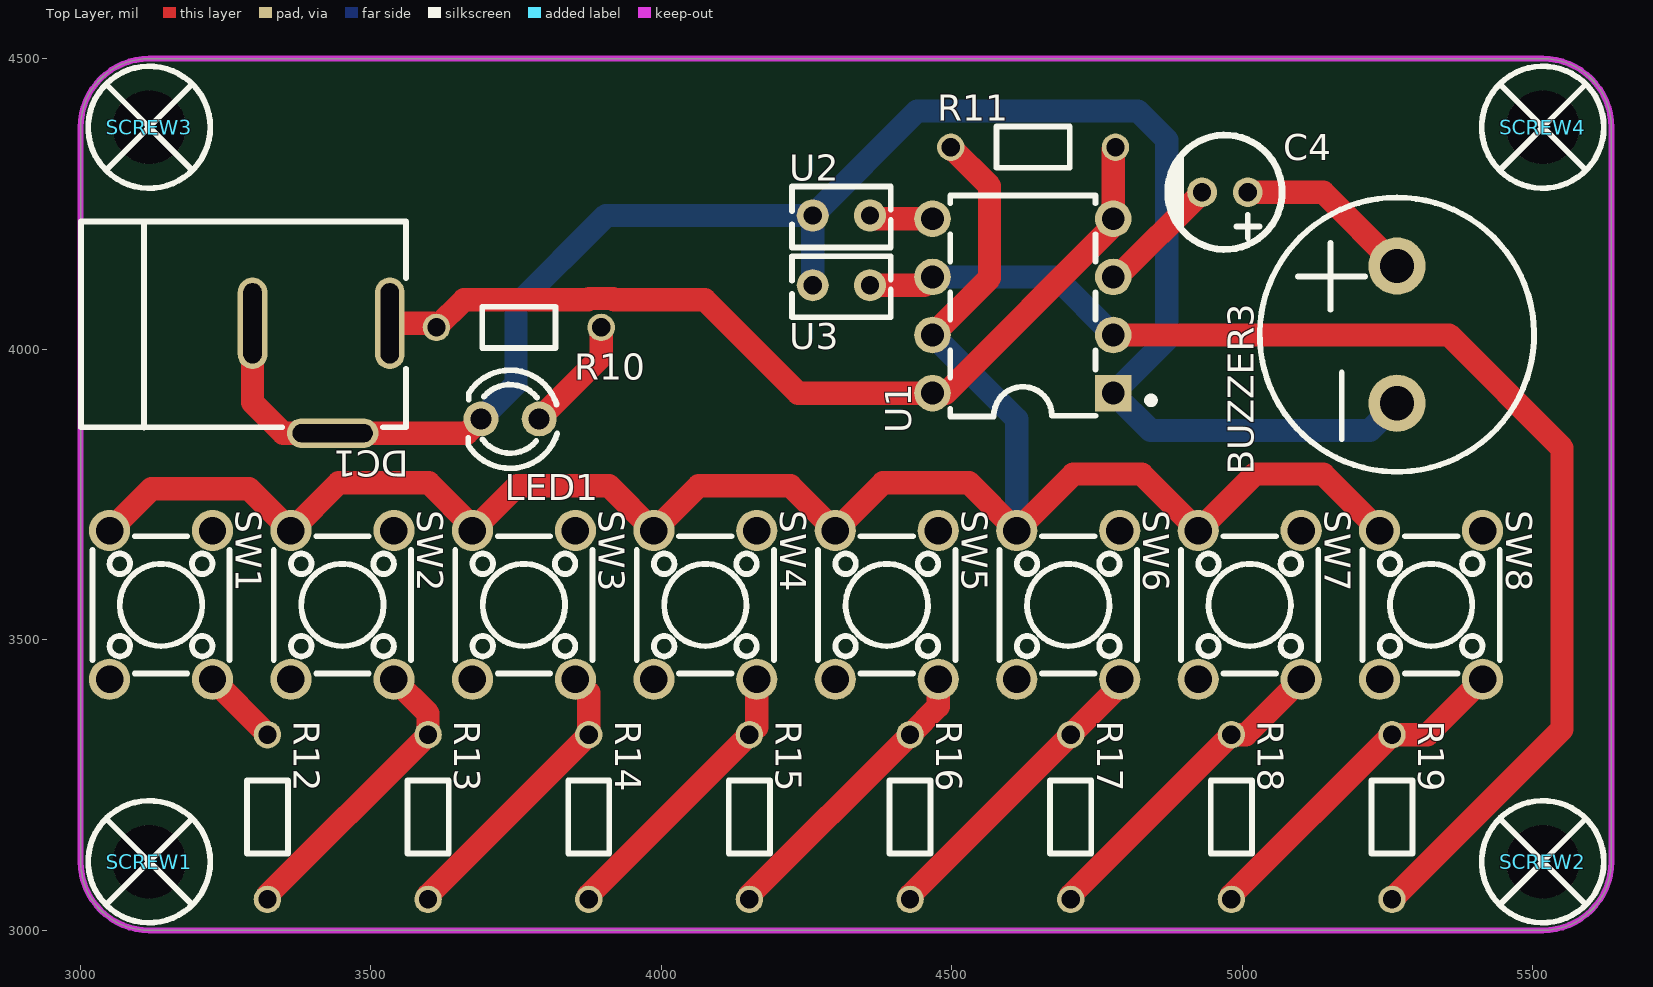
[diagram p0: Top Layer view]
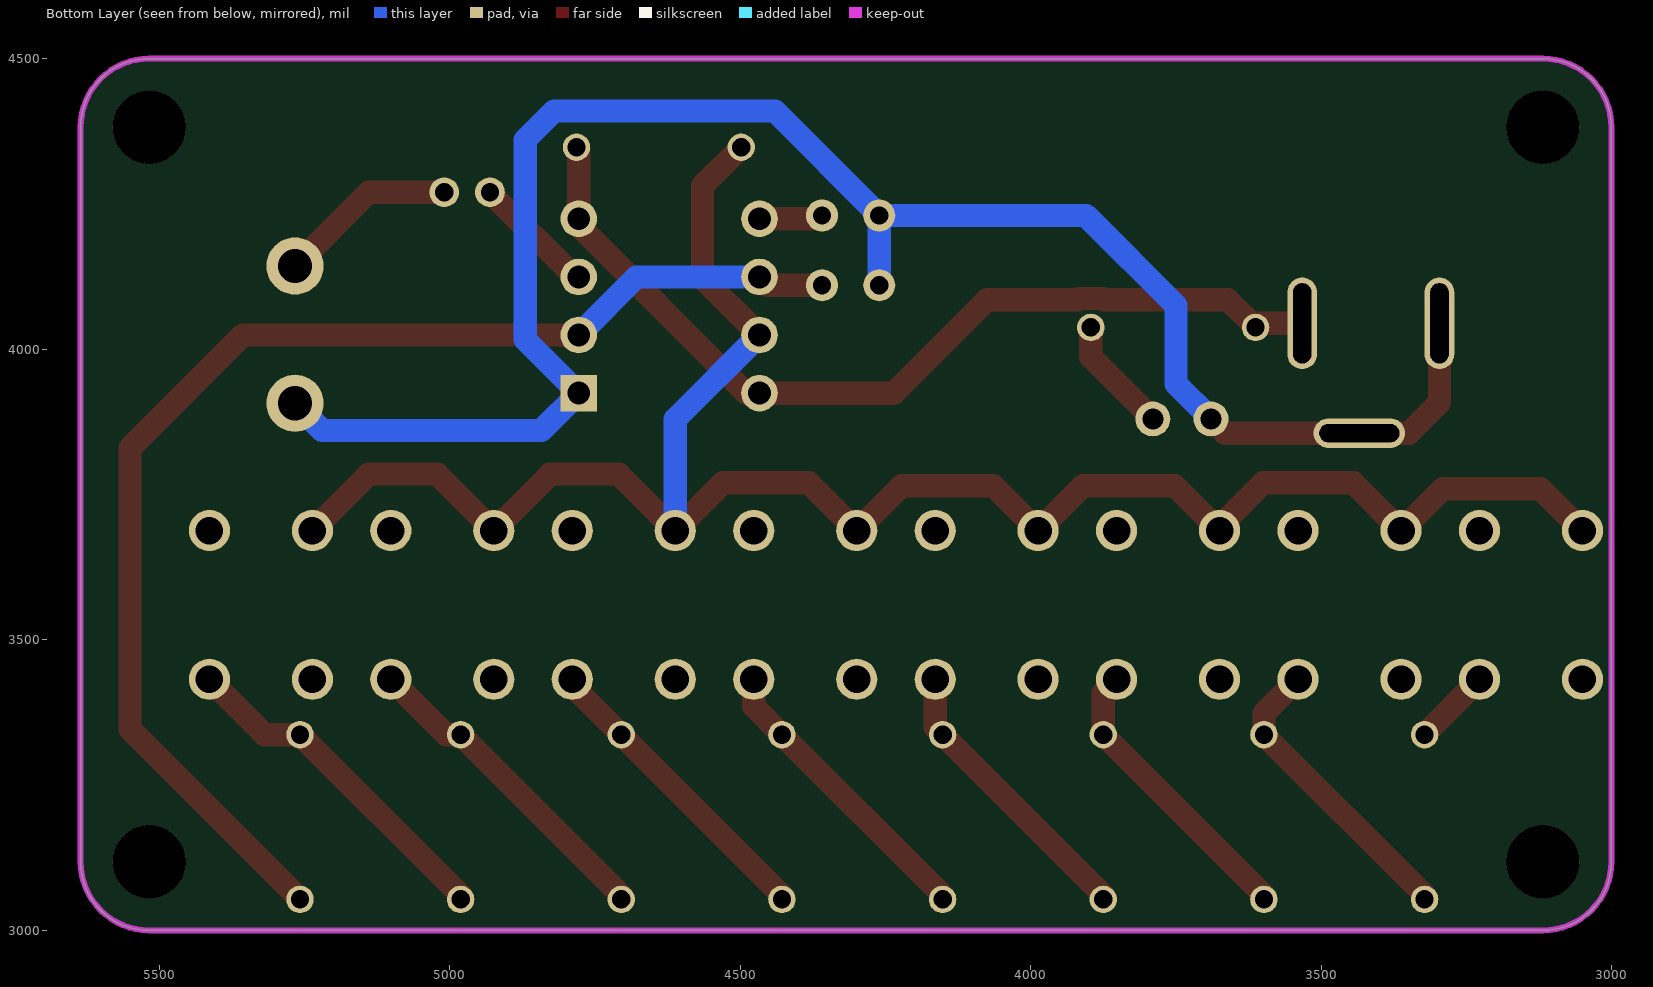
[diagram p1: Bottom Layer view, seen from below]
# Altium PCB MISC52051.pcbdoc
Units mil, origin at the board's own origin, x right, y up, seen from the top; angles counter-clockwise.
Board outline 2634.02 x 1500 mil, 2 copper layers (Top Layer, Bottom Layer), stack 62.206 mil thick; 29 components, 16 nets, 77 pads, 0 vias.

## Layer stack, top to bottom
Top Solder Mask Layer: solder mask 0.394, Dk 3.3
Top Layer: signal copper 1.379
Dielectric1: surface 59.449, FR4, Dk 4.5
Bottom Layer: signal copper 1.378
Bottom Solder Mask Layer: solder mask 0.394, Dk 3.3

## Board outline
3119.09,4500 ccw(c3119.09,4381.89) 3000.98,4381.89 3000.98,3118.11 ccw(c3119.09,3118.11) 3119.09,3000 5516.89,3000 ccw(c5516.89,3118.11) 5635,3118.11 5635,4381.89 ccw(c5516.89,4381.89) 5516.89,4500

## Design rules (kind name [scope] priority, off if disabled: settings)
BoardOutlineClearance copperThickness2oz_1 [All] p2 off: genericclearance=7.99 ignorepadtopadclearanceinfootprint=FALSE except(0: Arc-SplitContinuation Track-SplitContinuation SMDPad-SplitContinuation THPad-SplitContinuation Via-SplitContinuation Fill-SplitContinuation Region-SplitContinuation Poly-SplitContinuation Text-SplitContinuation Hole-SplitContinuation; 5.98: Arc-CutoutEdge Track-CutoutEdge SMDPad-CutoutEdge THPad-CutoutEdge Via-CutoutEdge Text-CutoutEdge; 6.9: Hole-OutlineEdge Hole-CutoutEdge; 10: Poly-OutlineEdge Poly-CutoutEdge; 11.81: Arc-OutlineEdge Track-OutlineEdge SMDPad-OutlineEdge THPad-OutlineEdge Via-OutlineEdge Fill-OutlineEdge Region-OutlineEdge Text-OutlineEdge Fill-CutoutEdge Region-CutoutEdge)
BoardOutlineClearance Plane_innerPlane_1 [All] p4 off: genericclearance=4.02 ignorepadtopadclearanceinfootprint=FALSE except(0: Arc-SplitContinuation Track-SplitContinuation SMDPad-SplitContinuation THPad-SplitContinuation Via-SplitContinuation Fill-SplitContinuation Region-SplitContinuation Poly-SplitContinuation Text-SplitContinuation Hole-SplitContinuation; 5.98: Arc-CutoutEdge Track-CutoutEdge SMDPad-CutoutEdge THPad-CutoutEdge Via-CutoutEdge Text-CutoutEdge; 6.9: Hole-OutlineEdge Hole-CutoutEdge; 10: Poly-OutlineEdge Poly-CutoutEdge; 11.81: Arc-OutlineEdge Track-OutlineEdge SMDPad-OutlineEdge THPad-OutlineEdge Via-OutlineEdge Fill-OutlineEdge Region-OutlineEdge Text-OutlineEdge Fill-CutoutEdge Region-CutoutEdge)
BoardOutlineClearance Copper_copperRegion_1 [All] p6 off: genericclearance=4.02 ignorepadtopadclearanceinfootprint=FALSE except(0: Arc-SplitContinuation Track-SplitContinuation SMDPad-SplitContinuation THPad-SplitContinuation Via-SplitContinuation Fill-SplitContinuation Region-SplitContinuation Poly-SplitContinuation Text-SplitContinuation Hole-SplitContinuation; 5.98: Arc-CutoutEdge Track-CutoutEdge SMDPad-CutoutEdge THPad-CutoutEdge Via-CutoutEdge Text-CutoutEdge; 6.9: Hole-OutlineEdge Hole-CutoutEdge; 10: Poly-OutlineEdge Poly-CutoutEdge; 11.81: Arc-OutlineEdge Track-OutlineEdge SMDPad-OutlineEdge THPad-OutlineEdge Via-OutlineEdge Fill-OutlineEdge Region-OutlineEdge Text-OutlineEdge Fill-CutoutEdge Region-CutoutEdge)
BoardOutlineClearance copperThickness1oz_1 [All] p8: genericclearance=4.02 ignorepadtopadclearanceinfootprint=FALSE except(0: Arc-SplitContinuation Track-SplitContinuation SMDPad-SplitContinuation THPad-SplitContinuation Via-SplitContinuation Fill-SplitContinuation Region-SplitContinuation Poly-SplitContinuation Text-SplitContinuation Hole-SplitContinuation; 5.98: Arc-CutoutEdge Track-CutoutEdge SMDPad-CutoutEdge THPad-CutoutEdge Via-CutoutEdge Text-CutoutEdge; 6.9: Hole-OutlineEdge Hole-CutoutEdge; 10: Poly-OutlineEdge Poly-CutoutEdge; 11.81: Arc-OutlineEdge Track-OutlineEdge SMDPad-OutlineEdge THPad-OutlineEdge Via-OutlineEdge Fill-OutlineEdge Region-OutlineEdge Text-OutlineEdge Fill-CutoutEdge Region-CutoutEdge)
Clearance copperThickness2oz [All] p1 off: gap=7.99 ignorepadtopadclearanceinfootprint=FALSE except(5.98: SMDPad-Track SMDPad-SMDPad THPad-Track SMDPad-THPad THPad-THPad Track-Via SMDPad-Via THPad-Via Via-Via Fill-SMDPad Region-SMDPad Fill-THPad Region-THPad Fill-Via Region-Via Fill-Fill Fill-Region Region-Region Arc-Track Arc-SMDPad Arc-THPad Arc-Via Fill-Arc Region-Arc Arc-Arc Text-Track SMDPad-Text Text-THPad Text-Via Fill-Text Region-Text Arc-Text Text-Text; 6.9: Hole-Track Hole-SMDPad Hole-THPad Hole-Via Fill-Hole Region-Hole Hole-Arc Hole-Text; 10: Poly-Track Poly-SMDPad Poly-THPad Poly-Via Poly-Fill Poly-Region Poly-Poly Poly-Arc Poly-Text Poly-Hole; 11.81: Fill-Track Region-Track)
Clearance Plane_innerPlane [All] p3 off: gap=4.02 ignorepadtopadclearanceinfootprint=FALSE except(5.98: SMDPad-Track SMDPad-SMDPad THPad-Track SMDPad-THPad THPad-THPad Track-Via SMDPad-Via THPad-Via Via-Via Fill-SMDPad Region-SMDPad Fill-THPad Region-THPad Fill-Via Region-Via Fill-Fill Fill-Region Region-Region Arc-Track Arc-SMDPad Arc-THPad Arc-Via Fill-Arc Region-Arc Arc-Arc Text-Track SMDPad-Text Text-THPad Text-Via Fill-Text Region-Text Arc-Text Text-Text; 6.9: Hole-Track Hole-SMDPad Hole-THPad Hole-Via Fill-Hole Region-Hole Hole-Arc Hole-Text; 10: Poly-Track Poly-SMDPad Poly-THPad Poly-Via Poly-Fill Poly-Region Poly-Poly Poly-Arc Poly-Text Poly-Hole; 11.81: Fill-Track Region-Track)
Clearance Copper_copperRegion [All] p5 off: gap=4.02 ignorepadtopadclearanceinfootprint=FALSE except(5.98: SMDPad-Track SMDPad-SMDPad THPad-Track SMDPad-THPad THPad-THPad Track-Via SMDPad-Via THPad-Via Via-Via Fill-SMDPad Region-SMDPad Fill-THPad Region-THPad Fill-Via Region-Via Fill-Fill Fill-Region Region-Region Arc-Track Arc-SMDPad Arc-THPad Arc-Via Fill-Arc Region-Arc Arc-Arc Text-Track SMDPad-Text Text-THPad Text-Via Fill-Text Region-Text Arc-Text Text-Text; 6.9: Hole-Track Hole-SMDPad Hole-THPad Hole-Via Fill-Hole Region-Hole Hole-Arc Hole-Text; 10: Poly-Track Poly-SMDPad Poly-THPad Poly-Via Poly-Fill Poly-Region Poly-Poly Poly-Arc Poly-Text Poly-Hole; 11.81: Fill-Track Region-Track)
Clearance copperThickness1oz [All] p7: gap=4.02 ignorepadtopadclearanceinfootprint=FALSE except(5.98: SMDPad-Track SMDPad-SMDPad THPad-Track SMDPad-THPad THPad-THPad Track-Via SMDPad-Via THPad-Via Via-Via Fill-SMDPad Region-SMDPad Fill-THPad Region-THPad Fill-Via Region-Via Fill-Fill Fill-Region Region-Region Arc-Track Arc-SMDPad Arc-THPad Arc-Via Fill-Arc Region-Arc Arc-Arc Text-Track SMDPad-Text Text-THPad Text-Via Fill-Text Region-Text Arc-Text Text-Text; 6.9: Hole-Track Hole-SMDPad Hole-THPad Hole-Via Fill-Hole Region-Hole Hole-Arc Hole-Text; 10: Poly-Track Poly-SMDPad Poly-THPad Poly-Via Poly-Fill Poly-Region Poly-Poly Poly-Arc Poly-Text Poly-Hole; 11.81: Fill-Track Region-Track)
DiffPairsRouting differentialPair [All] p1: maxlimit=6 minlimit=6 mostfreqgap=6 toplayer_minwidth=5 toplayer_prefwidth=10 toplayer_maxwidth=100 toplayer_mingap=6 toplayer_prefgap=6 toplayer_maxgap=6 bottomlayer_minwidth=5 bottomlayer_prefwidth=10 bottomlayer_maxwidth=100 bottomlayer_mingap=6 bottomlayer_prefgap=6 bottomlayer_maxgap=6 maxuncoupledlength=10
HoleToHoleClearance otherClearance [All] p1: gap=11.81 allowstackedmicrovias=TRUE
Length netLength [All] p1: minlimit=0 maxlimit=0
PasteMaskExpansion pasteMaskExpansion [All] p1: expansion=0
PlaneConnect innerPlane [All] p1: planeconnectstyle=Relief reliefexpansion=20 reliefentries=4 reliefconductorwidth=10 reliefairgap=10
PolygonConnect copperRegion [All] p1: connectstyle=Relief reliefconductorwidth=10 reliefentries=4 polygonreliefangle="90 Angle" airgapwidth=10 via.connectstyle=Relief via.reliefconductorwidth=10 via.reliefentries=4 via.polygonreliefangle="90 Angle" via.airgapwidth=10
RoutingVias viaSize [All] p1: holewidth=12.01 width=24.02 viastyle="Through Hole" minholewidth=11.81 minwidth=19.68 maxholewidth=248.03 maxwidth=393.7
SolderMaskExpansion solderMaskExpansion [IsVia] p1: expansion=-1000 istentingtop=TRUE
SolderMaskExpansion solderMaskExpansion [All] p2: expansion=2 istentingtop=FALSE
Width copperThickness2oz_2 [All] p1 off: maxlimit=100 minlimit=8 preferedwidth=10
Width copperThickness1oz_2 [All] p2: maxlimit=100 minlimit=5 preferedwidth=10

## Components (designator, comment, footprint, x,y, rotation, side; value= is the part's Value field where it differs from the comment)
BUZZER3 "buzzer" BUZ-TH_BD12.0-P6.00-D0.9-RD 5265.98,4025 r90 top
C4 "4.7uF" CAP-TH_BD5.0-P2.00-D0.8-FD 4970,4270 r180 top
DC1 "" DC-2.0 3410,4055 r180 top
LED1 "" LED_TH-3mm 3740,3880 r180 top
R10 "1kΩ" Res_1/8W 3755,4040 r180 top
R11 "1kΩ" Res_1/8W 4640,4345 r0 top
R12 "2kΩ" Res_1/8W 3320,3195 r270 top
R13 "2kΩ" Res_1/8W 3596.43,3195 r270 top
R14 "2kΩ" Res_1/8W 3872.86,3195 r270 top
R15 "2kΩ" Res_1/8W 4149.29,3195 r270 top
R16 "2kΩ" Res_1/8W 4425.71,3195 r270 top
R17 "2kΩ" Res_1/8W 4702.14,3195 r270 top
R18 "2kΩ" Res_1/8W 4978.57,3195 r270 top
R19 "2kΩ" Res_1/8W 5255,3195 r270 top
SCREW1 "" M3螺丝 3119.09,3118.11 r0 top
SCREW2 "" M3螺丝 5516.89,3118.11 r0 top
SCREW3 "" M3螺丝 3119.09,4381.89 r0 top
SCREW4 "" M3螺丝 5516.89,4381.89 r0 top
SW1 "" SW-TH_4P-L6.0-W6.0-P4.50-LS6.5 3139.36,3559.87 r270 top
SW2 "" SW-TH_4P-L6.0-W6.0-P4.50-LS6.5 3451.57,3559.87 r270 top
SW3 "" SW-TH_4P-L6.0-W6.0-P4.50-LS6.5 3763.77,3559.87 r270 top
SW4 "" SW-TH_4P-L6.0-W6.0-P4.50-LS6.5 4075.97,3559.87 r270 top
SW5 "" SW-TH_4P-L6.0-W6.0-P4.50-LS6.5 4388.18,3559.87 r270 top
SW6 "" SW-TH_4P-L6.0-W6.0-P4.50-LS6.5 4700.38,3559.87 r270 top
SW7 "" SW-TH_4P-L6.0-W6.0-P4.50-LS6.5 5012.58,3559.87 r270 top
SW8 "" SW-TH_4P-L6.0-W6.0-P4.50-LS6.5 5324.78,3559.87 r270 top
U1 "NE555" PDIP-8_L9.6-W6.4-P2.54-LS7.9-BL-1 4622.34,4074.34 r90 top
U2 "10nF" CAP-TH_L4.0-W2.5-P2.50-D0.5 4310,4230 r0 top
U3 "100nF" CAP-TH_L4.0-W2.5-P2.50-D0.5 4310,4110 r0 top

## Footprints (in the part's own frame and the unit in brackets; to place one, negate y for a bottom-side part, rotate by r counter-clockwise, add the part's x,y. Pads: shape width x height; smd on the part's side, far side on the other; paste and mask are expansions set on the pad)
BUZ-TH_BD12.0-P6.00-D0.9-RD [mm]
  round 2.5 hole 1.5 paste+0 mask+0.05: 1(-3,0) 2(3,0)
  silkscreen extent -5.99,-5.99 5.99,5.99
CAP-TH_BD5.0-P2.00-D0.8-FD [mm]
  round 1.3 hole 0.8: 1(-1,0) 2(1,0)
  silkscreen extent -2.5,-2.5 2.5,2.5
CAP-TH_L4.0-W2.5-P2.50-D0.5 [mm]
  round 1.4 hole 0.8 paste+0 mask+0.05: 1(-1.25,0) 2(1.25,0)
  silkscreen extent -2.16,-1.4 2.16,1.27
DC-2.0 [mil]
  oval 157.5x51.2 hole 31.5 slot 137.8 at 0 deg paste+0 mask+2: 2(-24.7,199.5)
  oval 51.2x157.5 hole 31.5 slot 137.8 at 90 deg paste+0 mask+2: 3(113.1,10.5) 4(-123.1,10.5)
  silkscreen extent -151,-165 408,190
LED_TH-3mm [mil]
  round 60 hole 36 paste+0 mask+2: 1(-50,0) 2(50,0)
  silkscreen extent -81,-84 72,85
M3螺丝 [mil]
  round 126 hole 126 paste+0 mask+4: 1(0,0)
  silkscreen extent -105,-105 105,105
PDIP-8_L9.6-W6.4-P2.54-LS7.9-BL-1 [mil]
  rect 63x63 hole 39.37: 1(-150,-155.51)
  round 63 hole 39.37: 2(-50,-155.51) 3(50,-155.51) 4(150,-155.51) 5(150,155.52) 6(50,155.52) 7(-50,155.52) 8(-150,155.52)
  silkscreen extent -190,-226 190,125
Res_1/8W [mil]
  round 47.2 hole 31.5 paste+0 mask+2: 1(-141.7,2.48) 2(141.7,2.48)
  silkscreen extent -63,-33 63,38
SW-TH_4P-L6.0-W6.0-P4.50-LS6.5 [mm]
  round 1.8 hole 1.2: 1(-3.25,2.25) 2(3.25,2.25) 3(-3.25,-2.25) 4(3.25,-2.25)
  silkscreen extent -3,-3 3,3

## Nets (pads, with @x,y where several pads share a name; then routed paths per layer and width w, separated by ;. In a path a pad name is that pad's centre, name@x,y a point inside that pad or via, vN(x,y) a via of type N, cw(c..) or ccw(c..) an arc to the next point about the centre after c; other vN are vias at no path point)
$1N233: R12.1 SW1.2 | length 134.4
  Top Layer w40: SW1.2 3322.48,3337.38 R12.1
$1N237: R12.2 R13.1 SW2.2 | length 517.5
  Top Layer w40: R12.2 3322.48,3060.27 R13.1 3598.91,3373.16 SW2.2
$1N293: R13.2 R14.1 SW3.2 | length 502.6
  Top Layer w40: R13.2 3598.91,3060.27 R14.1 3875.33,3408.93 SW3.2@3852.35,3431.92
$1N355: R14.2 R15.1 SW4.2 | length 498.4
  Top Layer w40: R14.2 3875.33,3060.27 R15.1 4164.55,3349.49 SW4.2
$1N416: R15.2 R16.1 SW5.2 | length 513.2
  Top Layer w40: R15.2 4151.76,3060.27 R16.1 4476.76,3385.26 SW5.2
$1N477: R16.2 R17.1 SW6.2 | length 528.1
  Top Layer w40: R16.2 4428.19,3060.27 R17.1 4788.96,3421.04 SW6.2
$1N538: R17.2 R18.1 SW7.2 | length 557.5
  Top Layer w40: R17.2 4704.62,3060.27 R18.1 5005.94,3336.7 SW7.2
$1N599: R18.2 R19.1 SW8.2 | length 593.2
  Top Layer w40: R18.2 4981.05,3060.27 R19.1 5318.15,3336.7 SW8.2
$1N660: R19.2 U1.2 U1.6 U3.2 | length 2216.5
  Top Layer w40: U3.2 4452.48,4110 U1.6 ; U1.2 5355.66,4024.34 5550,3830 5550,3345.82 R19.2
  Bottom Layer w40: U1.6 4677.85,4124.34 U1.2
$1N669: R11.1 SW1.3 SW2.3 SW3.3 SW4.3 SW5.3 SW6.3 SW7.3 SW8.3 U1.7 | length 3462.4
  Top Layer w40: SW1.3 3122.97,3760 3290.8,3760 SW2.3 3445.17,3770 3600,3770 3675.19,3694.81 SW3.3 3752.37,3765 3910.21,3765 SW4.3 4064.57,3765 4222.41,3765 SW5.3 4381.78,3770 4529.62,3770 SW6.3 4708.98,3785 4826.82,3785 SW7.3 5021.18,3785 5139.02,3785 SW8.3 ; U1.7 4565,4122.52 4565,4280.78 R11.1
  Bottom Layer w40: U1.7 4611.8,3879.37 SW6.3
$1N1188: U1.5 U2.2 | length 110
  Top Layer w40: U2.2 4364.87,4224.34 U1.5
$1N1258: C4.2 U1.3 | length 213.1
  Top Layer w40: U1.3 4784.97,4124.34 C4.2
$1N3814: BUZZER3.2 C4.1 | length 309.2
  Top Layer w40: C4.1 5139.09,4270 BUZZER3.2
$1N4636: LED1.1 R10.1 | length 201.7
  Top Layer w40: LED1.1 3896.7,3986.7 R10.1
+5V: DC1.4 R10.2 R11.2 U1.4 U1.8 | length 1591.3
  Top Layer w40: DC1.4 3606.32,4044.5 R10.2 3660.78,4085 3874.05,4085 3876.16,4087.11 3917.24,4087.11 3919.35,4085 4075,4085 4235.66,3924.34 U1.8 4489.34,3924.34 4777.85,4212.85 U1.4 4777.85,4343.62 R11.2
GND: BUZZER3.1 DC1.2 DC1.3 LED1.2 U1.1 U2.1 U3.1 | length 3188.8
  Top Layer w40: DC1.3 3296.9,3908.1 3349.5,3855.5 DC1.2 3665.5,3855.5 LED1.2
  Bottom Layer w40: LED1.2 3750,3940 3750,4075 3905,4230 U2.1 ; U3.1 U2.1 ; BUZZER3.1 5219.09,3860 4842.19,3860 U1.1 4870,4016.5 4870,4360 4820,4410 4440.79,4410 U2.1
pads on no net: SCREW1.1 SCREW2.1 SCREW3.1 SCREW4.1 SW1.1 SW1.4 SW2.1 SW2.4 SW3.1 SW3.4 SW4.1 SW4.4 SW5.1 SW5.4 SW6.1 SW6.4 SW7.1 SW7.4 SW8.1 SW8.4

## Keep-outs
Board Outline Layer:
  the board outline again, w10

## Silkscreen, mask and mechanical layers (free items; w line width, h text height)
Top Silkscreen Layer: